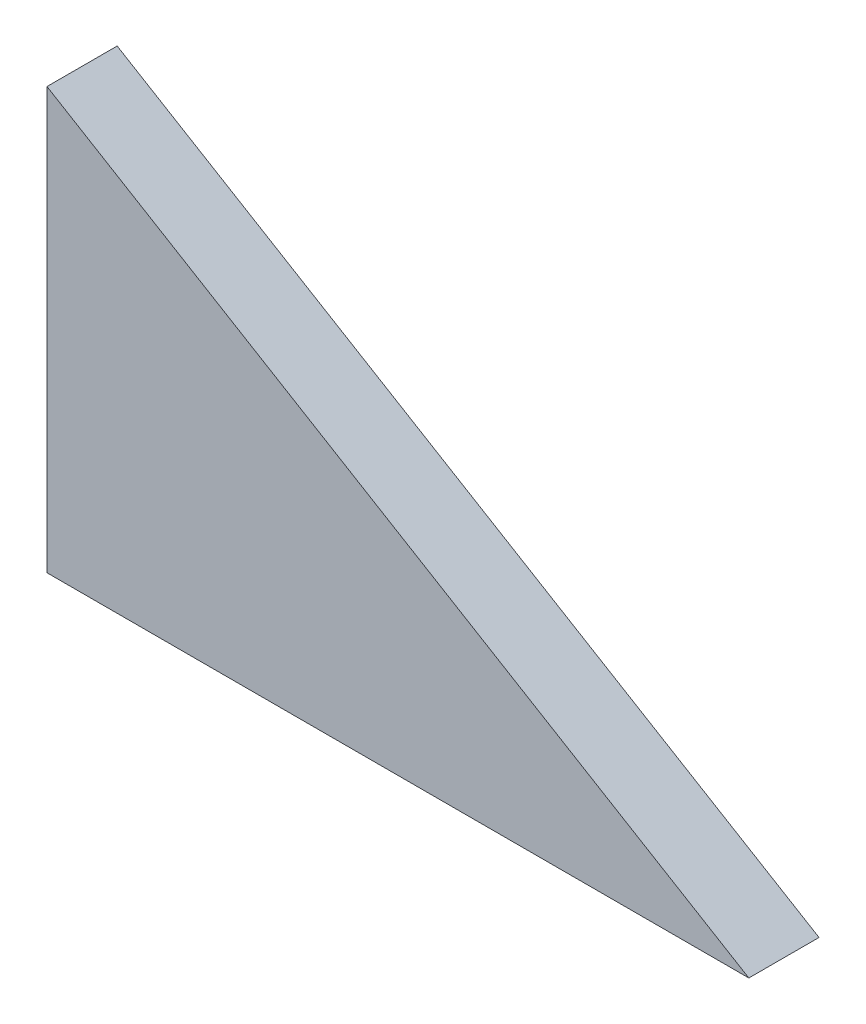
SolidWorks part; units mm, degrees
ref_plane "前视基准面" through (0, 0, 0) normal (0, 0, 1) x (1, 0, 0)
ref_plane "上视基准面" through (0, 0, 0) normal (0, 1, 0) x (1, 0, 0)
ref_plane "右视基准面" through (0, 0, 0) normal (1, 0, 0) x (0, 0, -1)
sketch "草图1" plane through (0, 0, 0) normal (0, 0, 1) x (1, 0, 0)
  line L0 (0, 0) -> (0, 30)
  line L1 (0, 0) -> (50, 0)
  line L2 (50, 0) -> (0, 30)
extrude "凸台-拉伸1" add sketch "草图1" along normal blind 5
